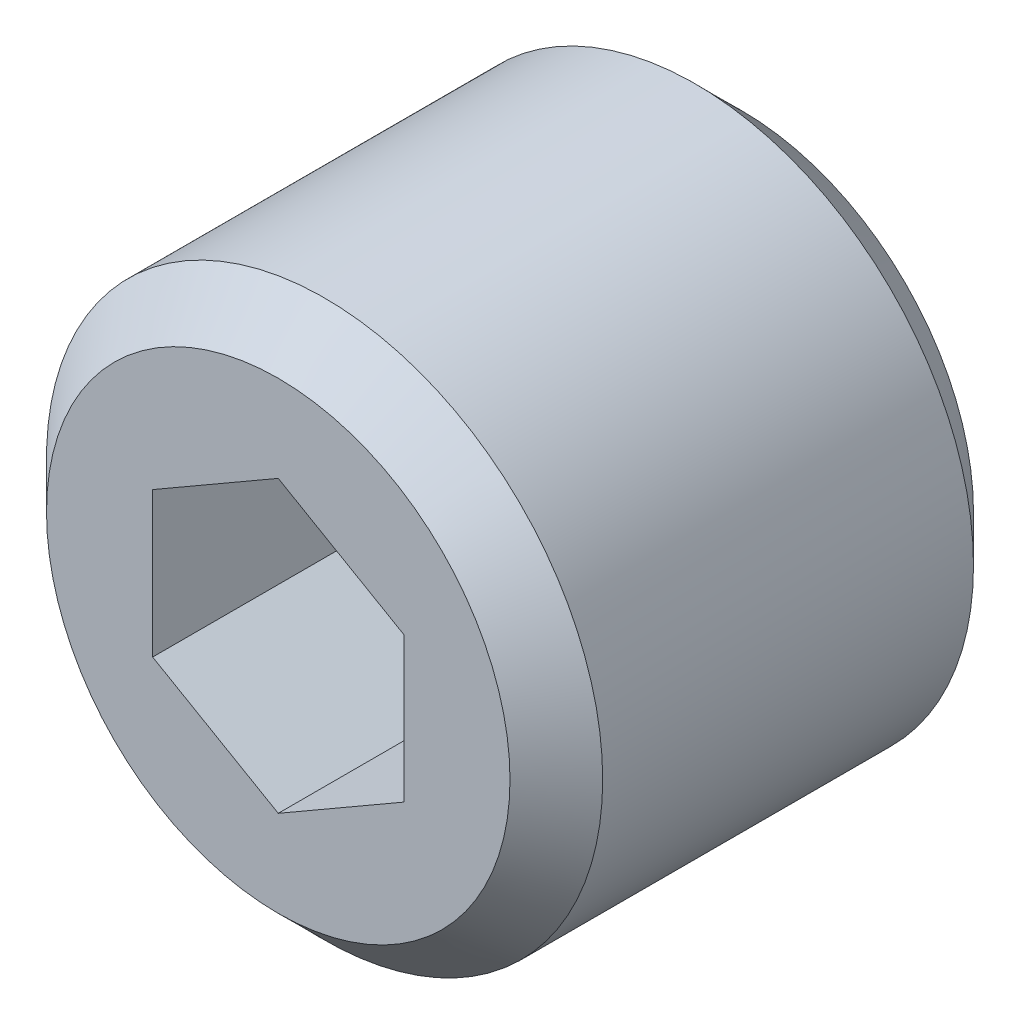
SolidWorks part; units mm, degrees
ref_plane "Front Plane" through (0, 0, 0) normal (0, 0, 1) x (1, 0, 0)
ref_plane "Top Plane" through (0, 0, 0) normal (0, 1, 0) x (1, 0, 0)
ref_plane "Right Plane" through (0, 0, 0) normal (1, 0, 0) x (0, 0, -1)
sketch "Sketch1" plane through (0, 0, 0) normal (0, 0, 1) x (1, 0, 0)
  circle A0 centre (0, 0) radius 6
  dimension "D1" = 12
extrude "Boss-Extrude1" add sketch "Sketch1" along normal blind 10
sketch "Sketch2" plane through (0, 0, 10) normal (0, 0, 1) x (1, 0, 0)
  line L1 (0, 3.1293) -> (-2.7101, 1.5646)
  line L2 (-2.7101, 1.5646) -> (-2.7101, -1.5646)
  line L3 (-2.7101, -1.5646) -> (0, -3.1293)
  line L4 (0, -3.1293) -> (2.7101, -1.5646)
  line L5 (2.7101, -1.5646) -> (2.7101, 1.5646)
  line L6 (2.7101, 1.5646) -> (0, 3.1293)
  circle A0 centre (0, 0) radius 2.7101 construction
extrude "Cut-Extrude1" cut sketch "Sketch2" against normal blind 5
chamfer "Chamfer1" distance 1 angle 45 2 edges at (6, 0, 10) (6, 0, 0)
